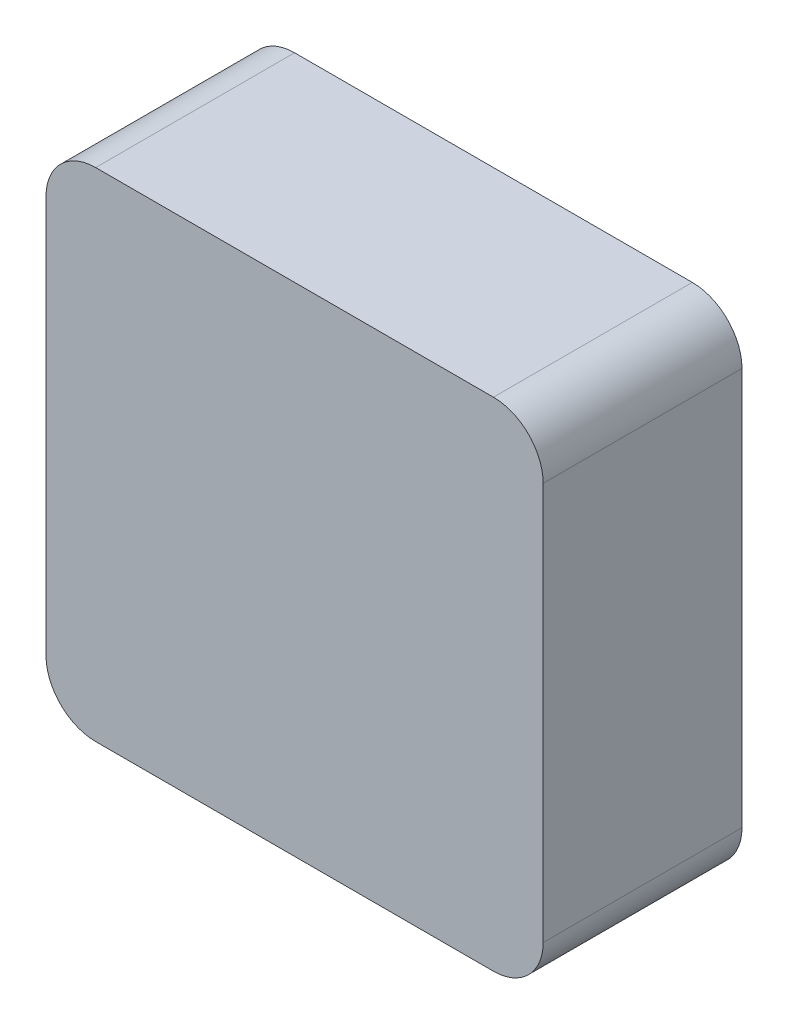
SolidWorks part; units mm, degrees
ref_plane "前视基准面" through (0, 0, 0) normal (0, 0, 1) x (1, 0, 0)
ref_plane "上视基准面" through (0, 0, 0) normal (0, 1, 0) x (1, 0, 0)
ref_plane "右视基准面" through (0, 0, 0) normal (1, 0, 0) x (0, 0, -1)
other "Configuration Table"
sketch "草图1" plane through (0, 0, 0) normal (0, 0, 1) x (1, 0, 0)
  line L1 (-50, -50) -> (50, -50)
  line L2 (-50, -50) -> (-50, 50)
  line L3 (-50, 50) -> (50, 50)
  line L4 (50, -50) -> (50, 50)
  line L5 (-50, -50) -> (50, 50) construction
  line L6 (-50, 50) -> (50, -50) construction
  circle A1 centre (0, 0) radius 37.5 construction
  point P0 (0, 0)
  dimension "D1" = 75
  dimension "D2" = 100
  dimension "D3" = 100
extrude "凸台-拉伸1" add sketch "草图1" along normal blind 40 contours L4 L3 L2 L1
sketch "草图2" plane through (0, 0, 0) normal (0, 0, -1) x (-1, 0, 0)
  circle A0 centre (0, 0) radius 37.5
  dimension "D1" = 75
extrude "切除-拉伸1" cut sketch "草图2" against normal blind 30 contours A0
fillet "圆角1" radius 10 4 edges at (50, -50, 20) (-50, -50, 20) (50, 50, 20) (-50, 50, 20)
